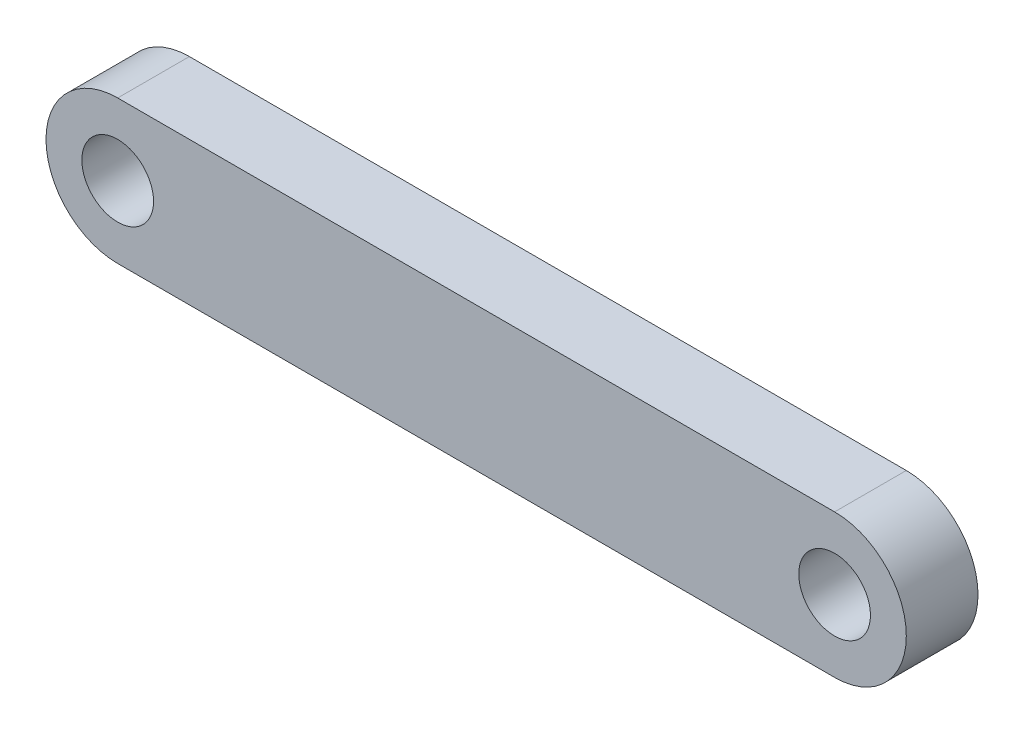
from build123d import *

# Parameters (mm, degrees)
SKETCH1_R           = 5
BOSS_EXTRUDE1_DEPTH = 10


with BuildPart() as part:
    # Sketch1 → Boss-Extrude1 (new body)
    with BuildSketch(Plane.XY):
        with BuildLine():
            Line((-25, 10), (75, 10))
            ThreePointArc((75, 10), (85, 0), (75, -10))
            Line((75, -10), (-25, -10))
            ThreePointArc((-25, -10), (-35, 0), (-25, 10))
        make_face()
        with Locations((75, 0)):
            Circle(SKETCH1_R, mode=Mode.SUBTRACT)
        with Locations((-25, 0)):
            Circle(SKETCH1_R, mode=Mode.SUBTRACT)
    extrude(amount=BOSS_EXTRUDE1_DEPTH)


solid = part.part
